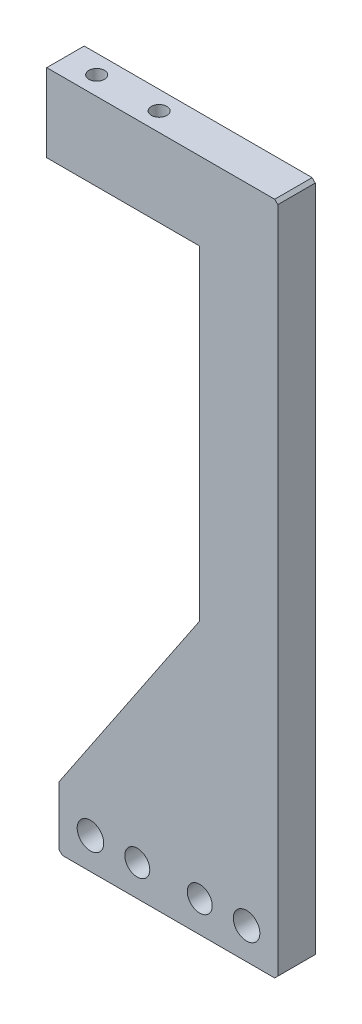
from build123d import *

# Parameters (mm, degrees)
EXTRUDE_1_DEPTH             = 12
HOLE_WIZARD_8_5_8_5_1_D     = 8.5
HOLE_WIZARD_8_5_8_5_1_DEPTH = 15.61
HOLE_WIZARD_8_5_8_5_1_TIP   = 2.453738644
SKETCH_5_R                  = 4
CUT_EXTRUDE_1_DEPTH         = 12
HOLE_WIZARD_M6_1_D          = 5
HOLE_WIZARD_M6_1_DEPTH      = 25
CHAMFER_1_SIZE              = 1
CHAMFER_2_SIZE              = 1


with BuildPart() as part:
    # 草图1 → 凸台-拉伸1 (new body)
    with BuildSketch(Plane.XY):
        Polygon((74.869050236, -20), (4.869050236, -20), (4.869050236, 0), (49.869050236, 67.029820029), (49.869050236, 171), (0.869050236, 171), (0.869050236, 196), (74.869050236, 196), align=None)
    extrude(amount=-EXTRUDE_1_DEPTH)

    # Ø8.5 (8.5) 直径孔1
    with Locations(Plane.XY):
        with Locations((64.869050236, -10), (14.869050236, -10)):
            Hole(HOLE_WIZARD_8_5_8_5_1_D / 2, depth=HOLE_WIZARD_8_5_8_5_1_DEPTH)
            with Locations((0, 0, -(HOLE_WIZARD_8_5_8_5_1_DEPTH + HOLE_WIZARD_8_5_8_5_1_TIP / 2))):  # 120° drill point
                Cone(0, HOLE_WIZARD_8_5_8_5_1_D / 2, HOLE_WIZARD_8_5_8_5_1_TIP, mode=Mode.SUBTRACT)

    # 草图5 → 切除-拉伸1 (cut)
    with BuildSketch(Plane.XY):
        with Locations((29.869050236, -10)):
            Circle(SKETCH_5_R)
        with Locations((49.869050236, -10)):
            Circle(SKETCH_5_R)
    extrude(amount=-CUT_EXTRUDE_1_DEPTH, mode=Mode.SUBTRACT)

    # M6 螺纹孔1
    with Locations(Plane(origin=(0, 196, 0), x_dir=(1, 0, 0), z_dir=(0, 1, 0))):
        with Locations((10.869050236, 6), (30.869050236, 6)):
            Hole(HOLE_WIZARD_M6_1_D / 2, depth=HOLE_WIZARD_M6_1_DEPTH)

    # 倒角1
    chamfer_1_edges = [part.edges().sort_by_distance(p)[0] for p in [
        (74.869050236, -20, -6),
        (74.869050236, 196, -6),
    ]]
    chamfer(chamfer_1_edges, length=CHAMFER_1_SIZE)

    # 倒角2
    chamfer_2_edges = [part.edges().sort_by_distance(p)[0] for p in [
        (4.869050236, -20, -6),
    ]]
    chamfer(chamfer_2_edges, length=CHAMFER_2_SIZE)


solid = part.part
